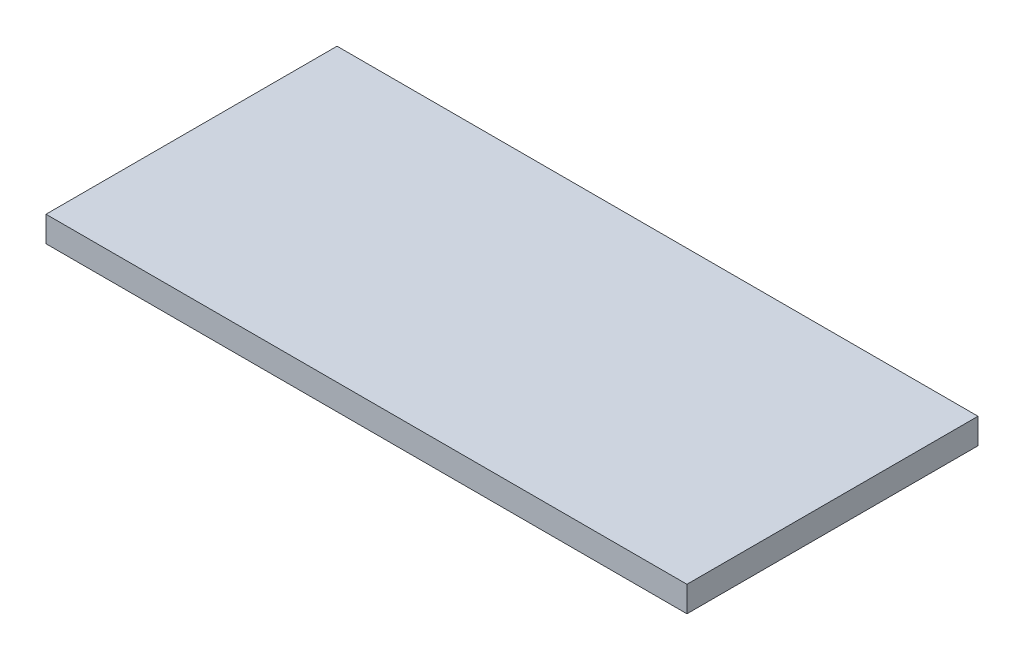
from build123d import *

# Parameters (mm, degrees)
EXTRUDE_THIN1_DEPTH = 500
SKETCH3_W           = 455
SKETCH3_H           = 40
EXTRUDE1_DEPTH      = 1
SKETCH7_W           = 455
SKETCH7_H           = 40
EXTRUDE3_DEPTH      = 1
SKETCH8_W           = 43
SKETCH8_H           = 1
CUT_EXTRUDE1_DEPTH  = 20
SKETCH9_R           = 2.75
CUT_EXTRUDE2_DEPTH  = 10


with BuildPart() as part:
    # Sketch2 → Extrude-Thin1 (new, symmetric)
    with BuildSketch(Plane(origin=(0, 0, 0), x_dir=(0, 0, -1), z_dir=(1, 0, 0))):
        Polygon((-22, -50), (-22, -40), (0, -40), (0, 0), (-455, 0), (-455, -40), (-454, -40), (-454, -1), (-1, -1), (-1, -39), (-23, -39), (-23, -50), align=None)
    extrude(amount=EXTRUDE_THIN1_DEPTH, both=True)

    # Sketch3 → Extrude1 (add)
    with BuildSketch(Plane(origin=(500, 0, 0), x_dir=(0, 0, -1), z_dir=(1, 0, 0))):
        with Locations((-227.5, -20)):
            Rectangle(SKETCH3_W, SKETCH3_H)
    extrude(amount=EXTRUDE1_DEPTH)

    # Sketch7 → Extrude3 (add)
    with BuildSketch(Plane.ZY.offset(500)):
        with Locations((227.5, -20)):
            Rectangle(SKETCH7_W, SKETCH7_H)
    extrude(amount=EXTRUDE3_DEPTH)

    # Sketch8 → Cut-Extrude1 (cut)
    with BuildSketch(Plane.XZ.offset(50)):
        with Locations((478.5, 22.5)):
            Rectangle(SKETCH8_W, SKETCH8_H)
        with Locations((-478.5, 22.5)):
            Rectangle(SKETCH8_W, SKETCH8_H)
    extrude(amount=-CUT_EXTRUDE1_DEPTH, mode=Mode.SUBTRACT)

    # Sketch9 → Cut-Extrude2 (cut)
    with BuildSketch(Plane.XZ.offset(40)):
        with Locations(Location((491, 15, 0), (0, 0, 270))):
            Circle(SKETCH9_R)
        with Locations(Location((-491, 15, 0), (0, 0, 270))):
            Circle(SKETCH9_R)
    extrude(amount=-CUT_EXTRUDE2_DEPTH, mode=Mode.SUBTRACT)


solid = part.part
